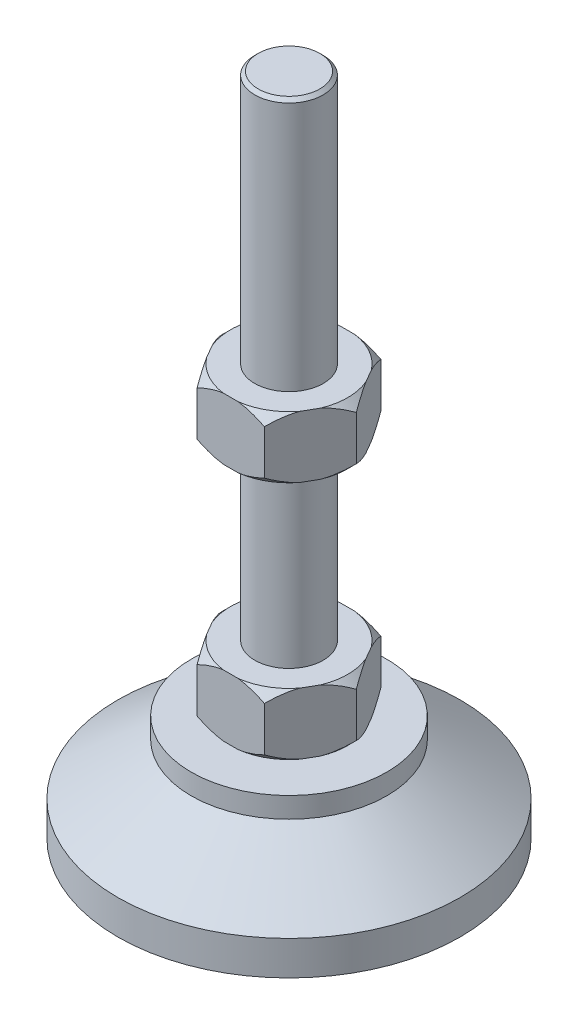
from build123d import *

# Parameters (mm, degrees)
SKETCH_2_R          = 28.577779899
EXTRUDE_1_DEPTH     = 6
SKETCH_4_R          = 24.484212217
CUT_EXTRUDE_5_DEPTH = 88
CHAMFER_1_SIZE      = 1


with BuildPart() as part:
    # 草图1 → 旋转1 (revolve)
    with BuildSketch(Plane.XY, mode=Mode.PRIVATE) as revolve_1_sk:
        Polygon((10, 169.340745793), (10, 95.340745793), (19.65, 95.340745793), (19.65, 77.340745793), (10, 77.340745793), (10, 25.340745793), (19.65, 25.340745793), (19.65, 7.340745793), (10, 7.340745793), (10, 0.340745793), (28.577779899, 0.340745793), (50, -14.659254207), (50, -24.659254207), (0, -24.659254207), (0, 169.340745793), align=None)
    revolve(revolve_1_sk.sketch.rotate(Axis((0, -29.818093999, 0), (0, 1, 0)), 90), axis=Axis((0, -29.818093999, 0), (0, 1, 0)))

    # 草图2 → 凸台-拉伸1 (add)
    with BuildSketch(Plane(origin=(0, 0.340745793, 0), x_dir=(1, 0, 0), z_dir=(0, 1, 0))):
        with Locations(Location((0, 0, 0), (0, 0, 270))):
            Circle(SKETCH_2_R)
    extrude(amount=EXTRUDE_1_DEPTH)

    # 草图4 → 切除-拉伸5 (cut)
    with BuildSketch(Plane(origin=(0, 95.340745793, 0), x_dir=(1, 0, 0), z_dir=(0, 1, 0))):
        Circle(SKETCH_4_R)
        Polygon((19.65, 0), (9.825, 17.017399184), (-9.825, 17.017399184), (-19.65, 0), (-9.825, -17.017399184), (9.825, -17.017399184), align=None, mode=Mode.SUBTRACT)
    extrude(amount=-CUT_EXTRUDE_5_DEPTH, mode=Mode.SUBTRACT)

    # 草图5 → 切除-旋转1 (revolve, cut)
    with BuildSketch(Plane.XY):
        Polygon((-17.15, 95.340745793), (-19.65, 92.840745793), (-26.926915052, 99.124494225), (-16.245783772, 99.906767383), align=None)
        Polygon((-17.15, 77.340745793), (-19.65, 79.840745793), (-19.65, 76.234905644), align=None)
        Polygon((-17.15, 25.340745793), (-19.65, 22.840745793), (-41.601041536, 16.623626451), (-25.840347108, 26.762569484), align=None)
        Polygon((-19.65, 9.840745793), (-17.15, 7.340745793), (-28.367472728, 7.340745793), align=None)
    revolve(axis=Axis((0, 180.885465797, 0), (0, -1, 0)), mode=Mode.SUBTRACT)

    # 倒角1
    chamfer_1_edges = [part.edges().sort_by_distance(p)[0] for p in [
        (0, 169.340745793, 10),
    ]]
    chamfer(chamfer_1_edges, length=CHAMFER_1_SIZE)


solid = part.part
